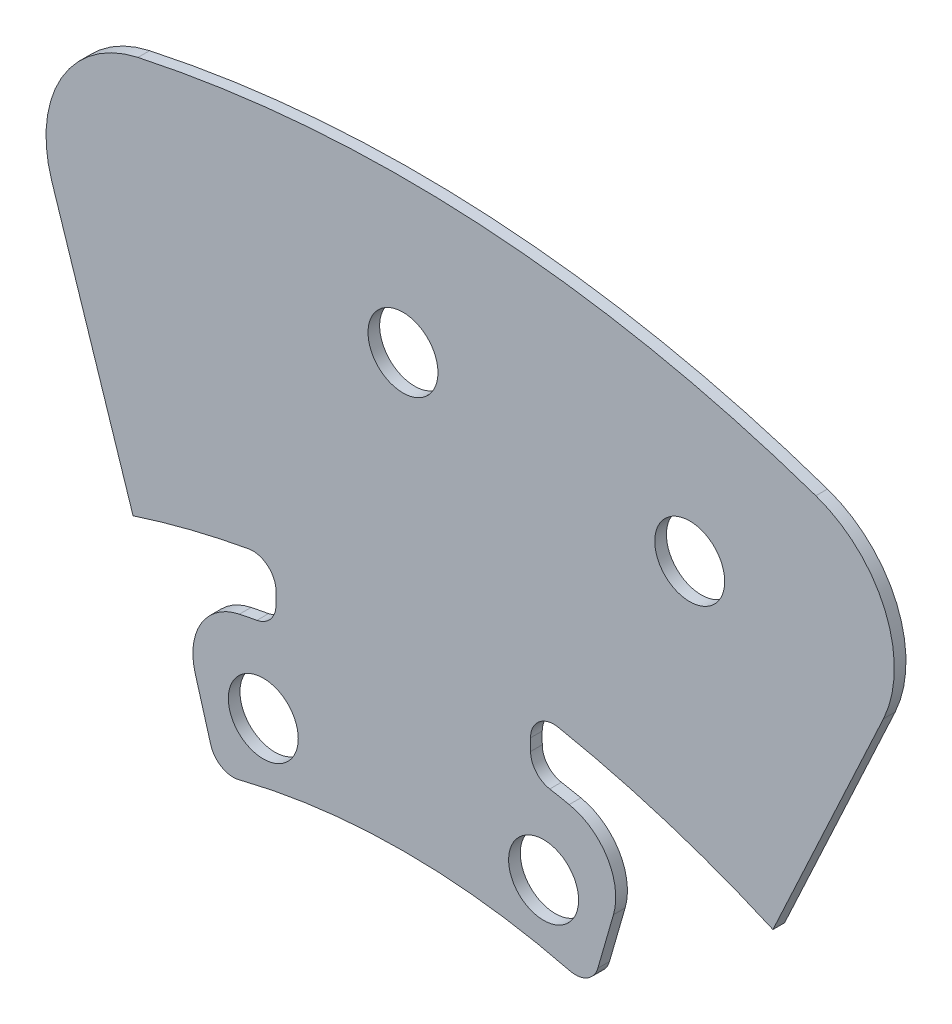
from build123d import *

# Parameters (mm, degrees)
SKETCH1_R           = 3
BOSS_EXTRUDE2_DEPTH = 1


with BuildPart() as part:
    # Sketch1 → Boss-Extrude2 (new body)
    with BuildSketch(Plane.XY):
        with BuildLine():
            Line((-23.148022373, -8.730243593), (-30.122846489, 12.649248922))
            ThreePointArc((-30.122846489, 12.649248922), (-29.288419203, 20.729586307), (-22.731208407, 25.524490657))
            ThreePointArc((-22.731208407, 25.524490657), (6.577970793, 27.774560597), (35.408236715, 22.038136022))
            ThreePointArc((35.408236715, 22.038136022), (41.345462771, 16.493997865), (41.208301592, 8.371848645))
            Line((41.208301592, 8.371848645), (31.728586192, -12.020940954))
            ThreePointArc((31.728586192, -12.020940954), (22.672300426, -8.599141601), (13.293379688, -6.198960674))
            ThreePointArc((13.293379688, -6.198960674), (11.656131568, -6.635918882), (10.941917146, -8.172607413))
            Line((10.941917146, -8.172607413), (10.944342154, -9.189079799))
            ThreePointArc((10.944342154, -9.189079799), (11.410804247, -10.468161557), (12.587919364, -11.152293875))
            ThreePointArc((12.587919364, -11.152293875), (13.423205338, -11.308812996), (14.256529596, -11.475461055))
            ThreePointArc((14.256529596, -11.475461055), (17.525943772, -13.786871862), (18.050961494, -17.7562604))
            Line((18.050961494, -17.7562604), (16.711120416, -22.40789263))
            ThreePointArc((16.711120416, -22.40789263), (15.785830822, -23.588348839), (14.300058147, -23.793573714))
            ThreePointArc((14.300058147, -23.793573714), (0.113320945, -22.031785702), (-14.073416257, -23.793573714))
            ThreePointArc((-14.073416257, -23.793573714), (-15.559188932, -23.588348839), (-16.484478526, -22.40789263))
            Line((-16.484478526, -22.40789263), (-17.824319603, -17.7562604))
            ThreePointArc((-17.824319603, -17.7562604), (-17.299301882, -13.786871862), (-14.029887705, -11.475461055))
            ThreePointArc((-14.029887705, -11.475461055), (-13.278530318, -11.324738612), (-12.525567944, -11.182250571))
            ThreePointArc((-12.525567944, -11.182250571), (-11.350088312, -10.495311954), (-10.886679055, -9.215120996))
            Line((-10.886679055, -9.215120996), (-10.886679055, -8.198645717))
            ThreePointArc((-10.886679055, -8.198645717), (-11.604557525, -6.663665462), (-13.242843438, -6.230614485))
            ThreePointArc((-13.242843438, -6.230614485), (-18.238041511, -7.311585647), (-23.148022373, -8.730243593))
        make_face()
        with Locations((12.060510133, -18.174977907)):
            Circle(SKETCH1_R, mode=Mode.SUBTRACT)
        with Locations((-11.981406179, -18.203656377)):
            Circle(SKETCH1_R, mode=Mode.SUBTRACT)
        with Locations((0, 14.968146711)):
            Circle(SKETCH1_R, mode=Mode.SUBTRACT)
        with Locations((24.591653109, 11.76043213)):
            Circle(SKETCH1_R, mode=Mode.SUBTRACT)
    extrude(amount=BOSS_EXTRUDE2_DEPTH)


solid = part.part
